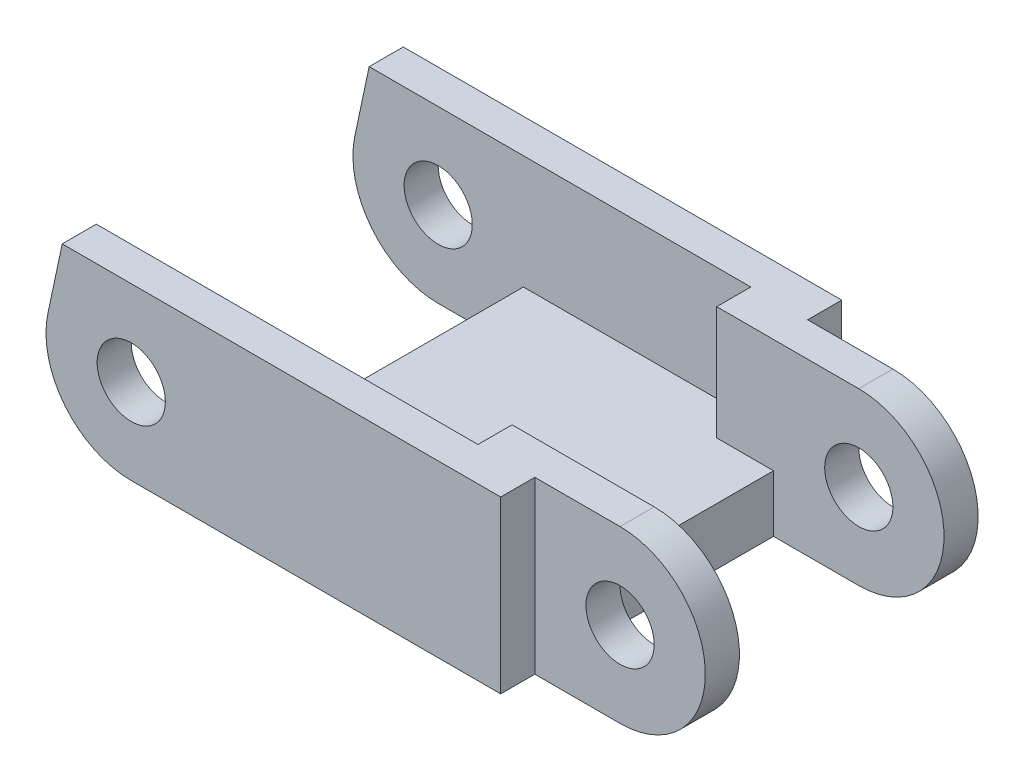
SolidWorks part; units mm, degrees
ref_plane "Front Plane" through (0, 0, 0) normal (0, 0, 1) x (1, 0, 0)
ref_plane "Top Plane" through (0, 0, 0) normal (0, 1, 0) x (1, 0, 0)
ref_plane "Right Plane" through (0, 0, 0) normal (1, 0, 0) x (0, 0, -1)
other "Configuration Table"
sketch "Sketch1" plane through (0, 0, 0) normal (0, 0, 1) x (1, 0, 0)
  line L0 (1.9256, 9.0593) -> (3.1883, 15)
  line L1 (3.1883, 15) -> (49.2617, 15)
  line L3 (49.2617, 0) -> (9.2617, 0)
  arc A0 (1.9256, 9.0593) -> (9.2617, 0) centre (9.2617, 7.5) ccw
  circle A1 centre (9.2617, 7.5) radius 3
  arc A2 (49.2617, 0) -> (49.2617, 15) centre (49.2617, 7.5) ccw
  circle A3 centre (49.2617, 7.5) radius 3
  point P7 (0, 0)
  dimension "D2" = 7.5
  dimension "D3" = 6
  dimension "D6" = 6
  dimension "D1" = 78
  dimension "D4" = 15
  dimension "D5" = 40
extrude "Boss-Extrude1" add sketch "Sketch1" along normal blind 30
sketch "Sketch2" plane through (0, 15, 0) normal (0, 1, 0) x (1, 0, 0)
  line L0 (1.7617, 0) -> (1.7617, -30) construction
  line L1 (-13.2383, -3) -> (16.7617, -3)
  line L2 (-13.2383, -3) -> (-13.2383, -27)
  line L3 (-13.2383, -27) -> (16.7617, -27)
  line L4 (16.7617, -3) -> (16.7617, -27)
  line L5 (1.7617, -27) -> (1.7617, -3) construction
  line L6 (-13.2383, -15) -> (16.7617, -15) construction
  line L7 (1.7617, -15) -> (69.019, -15) construction
  line L8 (41.7617, 3) -> (71.7617, 3)
  line L9 (41.7617, 3) -> (41.7617, -3)
  line L10 (41.7617, -3) -> (71.7617, -3)
  line L11 (71.7617, 3) -> (71.7617, -3)
  line L12 (56.7617, -3) -> (56.7617, 3) construction
  line L13 (41.7617, 0) -> (71.7617, 0) construction
  line L14 (41.7617, -27) -> (71.7617, -27)
  line L15 (41.7617, -27) -> (41.7617, -33)
  line L16 (41.7617, -33) -> (71.7617, -33)
  line L17 (71.7617, -27) -> (71.7617, -33)
  line L18 (56.7617, -33) -> (56.7617, -27) construction
  line L19 (41.7617, -30) -> (71.7617, -30) construction
  point P0 (1.7617, -15)
  point P6 (56.7617, 0)
  point P10 (56.7617, -30)
  dimension "D1" = 15
  dimension "D2" = 15
  dimension "D3" = 24
  dimension "D4" = 15
  dimension "D5" = 24
extrude "Cut-Extrude1" cut sketch "Sketch2" against normal blind 30
sketch "Sketch3" plane through (0, 15, 0) normal (0, 1, 0) x (1, 0, 0)
  line L0 (16.7617, -27) -> (16.7617, -3) construction
  line L1 (-3.2383, -3) -> (36.7617, -3)
  line L2 (-3.2383, -3) -> (-3.2383, -27)
  line L3 (-3.2383, -27) -> (36.7617, -27)
  line L4 (36.7617, -3) -> (36.7617, -6)
  line L5 (16.7617, -27) -> (16.7617, -24) construction
  line L6 (-3.2383, -15) -> (36.7617, -15) construction
  line L7 (16.7617, -15) -> (16.7617, -3) construction
  line L8 (36.7617, -6) -> (65.3752, -6)
  line L10 (36.7617, -24) -> (65.3752, -24)
  line L11 (65.3752, -6) -> (65.3752, -24)
  line L13 (16.7617, -15) -> (65.3752, -15) construction
  line L14 (36.7617, -24) -> (36.7617, -27)
  point P0 (16.7617, -15)
  dimension "D1" = 20
  dimension "D2" = 24
  dimension "D3" = 18
extrude "Cut-Extrude2" cut sketch "Sketch3" against normal blind 10
sketch "Sketch4" plane through (0, 5, 0) normal (0, 1, 0) x (1, 0, 0)
  line L0 (56.3328, -24) -> (56.3328, -6) construction
  line L1 (70.9039, -24) -> (41.7617, -24)
  line L2 (70.9039, -24) -> (70.9039, -6)
  line L3 (70.9039, -6) -> (41.7617, -6)
  line L4 (41.7617, -24) -> (41.7617, -6)
  line L5 (56.3328, -6) -> (56.3328, -24) construction
  line L6 (70.9039, -15) -> (41.7617, -15) construction
  line L8 (41.7617, 0) -> (41.7617, -3) construction
  point P0 (56.3328, -15)
extrude "Cut-Extrude3" cut sketch "Sketch4" against normal blind 12
